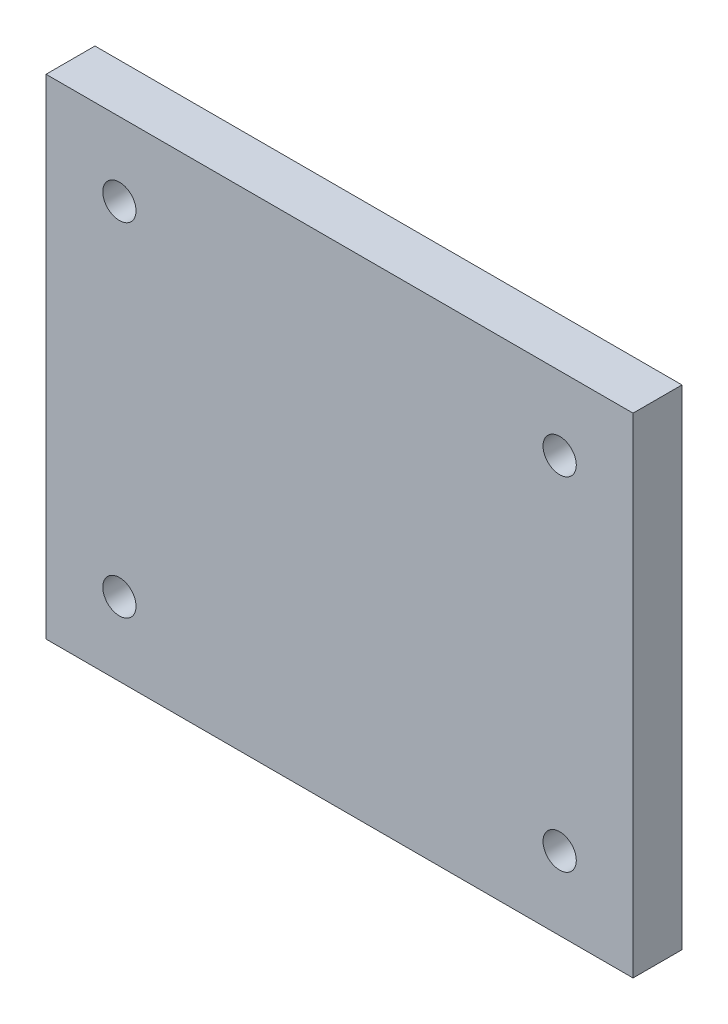
from build123d import *

# Parameters (mm, degrees)
SKETCH1_W             = 120
SKETCH1_H             = 100
BOSS_EXTRUDE1_DEPTH   = 10
M8_TAPPED_HOLE1_D     = 6.8
M8_TAPPED_HOLE1_DEPTH = 19.75
M8_TAPPED_HOLE1_TIP   = 2.042926105


with BuildPart() as part:
    # Sketch1 → Boss-Extrude1 (new body)
    with BuildSketch(Plane.XY):
        Rectangle(SKETCH1_W, SKETCH1_H)
    extrude(amount=BOSS_EXTRUDE1_DEPTH)

    # M8 Tapped Hole1
    with Locations(Plane.XY.offset(10)):
        with Locations((45, -35), (-45, -35), (-45, 35), (45, 35)):
            Hole(M8_TAPPED_HOLE1_D / 2, depth=M8_TAPPED_HOLE1_DEPTH)
            with Locations((0, 0, -(M8_TAPPED_HOLE1_DEPTH + M8_TAPPED_HOLE1_TIP / 2))):  # 118° drill point
                Cone(0, M8_TAPPED_HOLE1_D / 2, M8_TAPPED_HOLE1_TIP, mode=Mode.SUBTRACT)


solid = part.part
